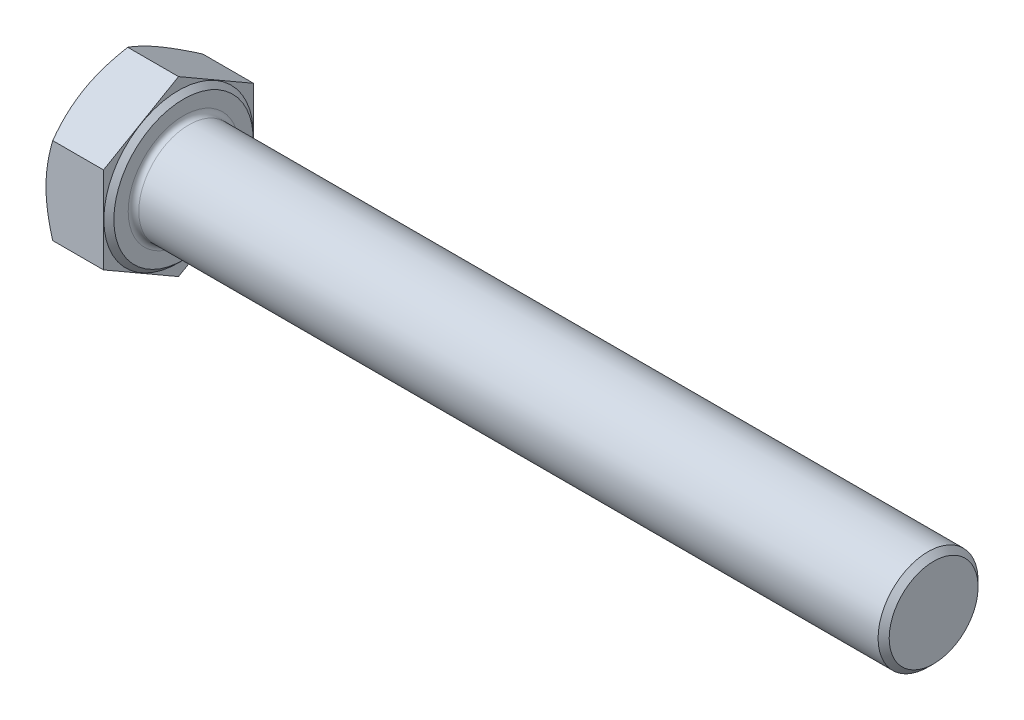
from build123d import *

# Parameters (mm, degrees)
BOSS_EXTRUDE1_DEPTH = 10
SKETCH4_R           = 26.75
SKETCH4_R_2         = 12
CUT_EXTRUDE1_DEPTH  = 1.25
CUT_EXTRUDE1_DRAFT  = -60
CHAMFER2_SIZE       = 0.888888889


with BuildPart() as part:
    # Sketch3 → Boss-Extrude1 (new body)
    with BuildSketch(Plane(origin=(0, 0, 0), x_dir=(0, 0, -1), z_dir=(1, 0, 0))):
        Polygon((12, 6.92820323), (0, 13.856406461), (-12, 6.92820323), (-12, -6.92820323), (0, -13.856406461), (12, -6.92820323), align=None)
    extrude(amount=BOSS_EXTRUDE1_DEPTH)


with BuildPart() as cut_extrude1_tool:
    # Sketch4 → Cut-Extrude1 (with draft: the straight prism first)
    with BuildSketch(Plane.ZY):
        Circle(SKETCH4_R)
        Circle(SKETCH4_R_2, mode=Mode.SUBTRACT)
    extrude(amount=-CUT_EXTRUDE1_DEPTH)
    # Cut-Extrude1: the draft: its side faces are tilted about the plane it starts from
    cut_extrude1_sides = [cut_extrude1_tool.faces().sort_by_distance(p)[0] for p in [
        (0.625, 0, -26.75),
        (0.625, 0, -12),
    ]]
    draft(cut_extrude1_sides, Plane.ZY, CUT_EXTRUDE1_DRAFT)


with BuildPart() as part_1:
    add(part.part)

    # Cut-Extrude1: cut by cut_extrude1_tool
    add(cut_extrude1_tool.part, mode=Mode.SUBTRACT)

    # Sketch5 → Revolve1 (revolve)
    with BuildSketch(Plane.XY, mode=Mode.PRIVATE) as revolve1_sk:
        with BuildLine():
            Line((10.85, 8), (130, 8))
            Line((130, 8), (130, 0))
            Line((130, 0), (10, 0))
            Line((10, 0), (10, 8.85))
            ThreePointArc((10, 8.85), (10.248959236, 8.248959236), (10.85, 8))
        make_face()
    revolve(revolve1_sk.sketch.rotate(Axis((10, 0, 0), (1, 0, 0)), 90), axis=Axis((10, 0, 0), (1, 0, 0)))

    # Chamfer2
    chamfer2_edges = [part_1.edges().sort_by_distance(p)[0] for p in [
        (130, 0, -8),
    ]]
    chamfer(chamfer2_edges, length=CHAMFER2_SIZE)

    # Sketch7 → Cut-Revolve1 (revolve, cut)
    with BuildSketch(Plane.XY, mode=Mode.PRIVATE) as cut_revolve1_sk:
        Polygon((10, 11.145), (9.2, 11.945), (9.2, 26.75), (10, 26.75), align=None)
    revolve(cut_revolve1_sk.sketch.rotate(Axis((0, 0, 0), (1, 0, 0)), 90), axis=Axis((0, 0, 0), (1, 0, 0)), mode=Mode.SUBTRACT)


solid = part_1.part
